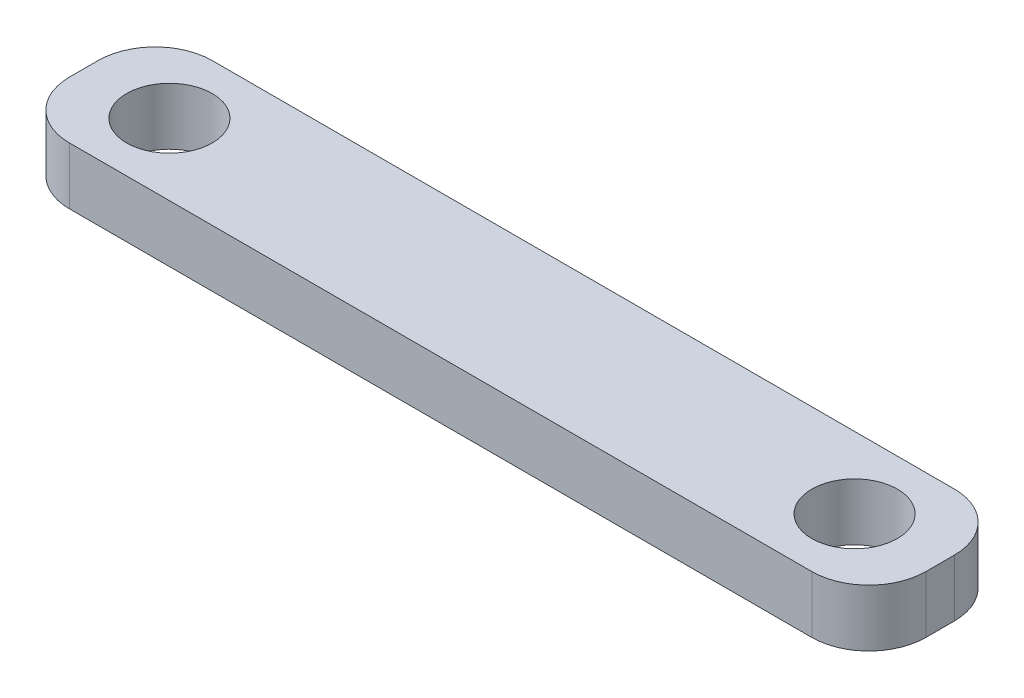
from build123d import *

# Parameters (mm, degrees)
SKETCH1_R           = 1.5
BOSS_EXTRUDE1_DEPTH = 2


with BuildPart() as part:
    # Sketch1 → Boss-Extrude1 (new body)
    with BuildSketch(Plane(origin=(0, 0, 0), x_dir=(1, 0, 0), z_dir=(0, 1, 0))):
        with BuildLine():
            Line((-13, -2.5), (13, -2.5))
            ThreePointArc((13, -2.5), (14.414213562, -1.914213562), (15, -0.5))
            Line((15, -0.5), (15, 0.5))
            ThreePointArc((15, 0.5), (14.414213562, 1.914213562), (13, 2.5))
            Line((13, 2.5), (-13, 2.5))
            ThreePointArc((-13, 2.5), (-14.414213562, 1.914213562), (-15, 0.5))
            Line((-15, 0.5), (-15, -0.5))
            ThreePointArc((-15, -0.5), (-14.414213562, -1.914213562), (-13, -2.5))
        make_face()
        with Locations(Location((12, 0, 0), (0, 0, 270))):
            Circle(SKETCH1_R, mode=Mode.SUBTRACT)
        with Locations(Location((-12, 0, 0), (0, 0, 270))):
            Circle(SKETCH1_R, mode=Mode.SUBTRACT)
    extrude(amount=BOSS_EXTRUDE1_DEPTH)


solid = part.part
